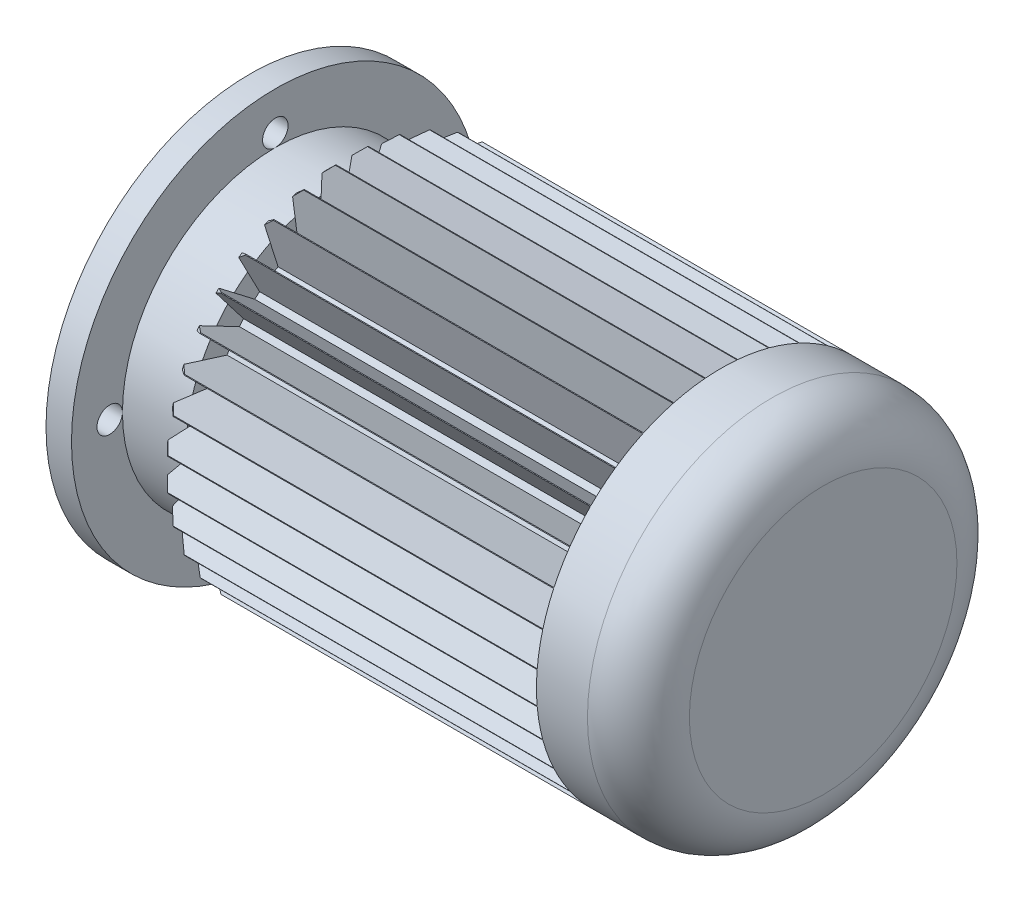
from build123d import *

# Parameters (mm, degrees)
FILLET_1_R               = 20
CHAMFER_1_SIZE           = 5
CUT_EXTRUDE_START        = -150
CUT_EXTRUDE_1_DEPTH      = 150
PATTERN_CIRCULAR_1_COUNT = 36
CUT_EXTRUDE_2_REACH      = 253.843
SKETCH_4_R               = 5
PATTERN_CIRCULAR_2_COUNT = 4


with BuildPart() as part:
    # 草图1 → 旋转1 (revolve)
    with BuildSketch(Plane.XY, mode=Mode.PRIVATE) as revolve_1_sk:
        Polygon((0, 0), (0, 55), (3.5, 55), (3.5, 80), (13.5, 80), (13.5, 60), (38.5, 60), (38.5, 72.5), (228.5, 72.5), (228.5, 0), align=None)
    revolve(revolve_1_sk.sketch.rotate(Axis((0, 0, 0), (1, 0, 0)), 90), axis=Axis((0, 0, 0), (1, 0, 0)))

    # 圆角1
    fillet_1_edges = [part.edges().sort_by_distance(p)[0] for p in [
        (228.5, 0, -72.5),
    ]]
    fillet(fillet_1_edges, radius=FILLET_1_R)

    # 倒角1
    chamfer_1_edges = [part.edges().sort_by_distance(p)[0] for p in [
        (38.5, 0, -72.5),
    ]]
    chamfer(chamfer_1_edges, length=CHAMFER_1_SIZE)

    # 草图3 → 切除-拉伸1 (cut)
    with BuildSketch(Plane.ZY.offset(-38.5).offset(CUT_EXTRUDE_START)):
        with BuildLine():
            Line((6.179636879, 72.236154992), (1.25, 50))
            Line((1.25, 50), (-1.25, 50))
            Line((-1.25, 50), (-6.179636879, 72.236154992))
            ThreePointArc((-6.179636879, 72.236154992), (0, 72.5), (6.179636879, 72.236154992))
        make_face()
    cut_extrude_1 = extrude(amount=CUT_EXTRUDE_1_DEPTH, mode=Mode.SUBTRACT)

    # 阵列(圆周)1: 切除-拉伸1 ×36 about axis
    pattern_circular_1_axis = Axis((0, 0, 0), (1, 0, 0))
    for i in range(1, PATTERN_CIRCULAR_1_COUNT):
        add(cut_extrude_1.rotate(pattern_circular_1_axis, i * 360 / PATTERN_CIRCULAR_1_COUNT), mode=Mode.SUBTRACT)

    # 草图4 → 切除-拉伸2 (cut, up to next)
    with BuildSketch(Plane.ZY.offset(-3.5), mode=Mode.PRIVATE) as cut_extrude_2_sk1:
        with Locations((0, 65)):
            Circle(SKETCH_4_R)
    cut_extrude_2_tool1 = extrude(cut_extrude_2_sk1.sketch, amount=-CUT_EXTRUDE_2_REACH, mode=Mode.PRIVATE) & part.part
    cut_extrude_2 = cut_extrude_2_tool1.solids().sort_by_distance((3.5, 65, 0))[0]
    add(cut_extrude_2, mode=Mode.SUBTRACT)

    # 阵列(圆周)2: 切除-拉伸2 ×4 about axis
    pattern_circular_2_axis = Axis((0, 0, 0), (1, 0, 0))
    for i in range(1, PATTERN_CIRCULAR_2_COUNT):
        add(cut_extrude_2.rotate(pattern_circular_2_axis, i * 360 / PATTERN_CIRCULAR_2_COUNT), mode=Mode.SUBTRACT)


solid = part.part
